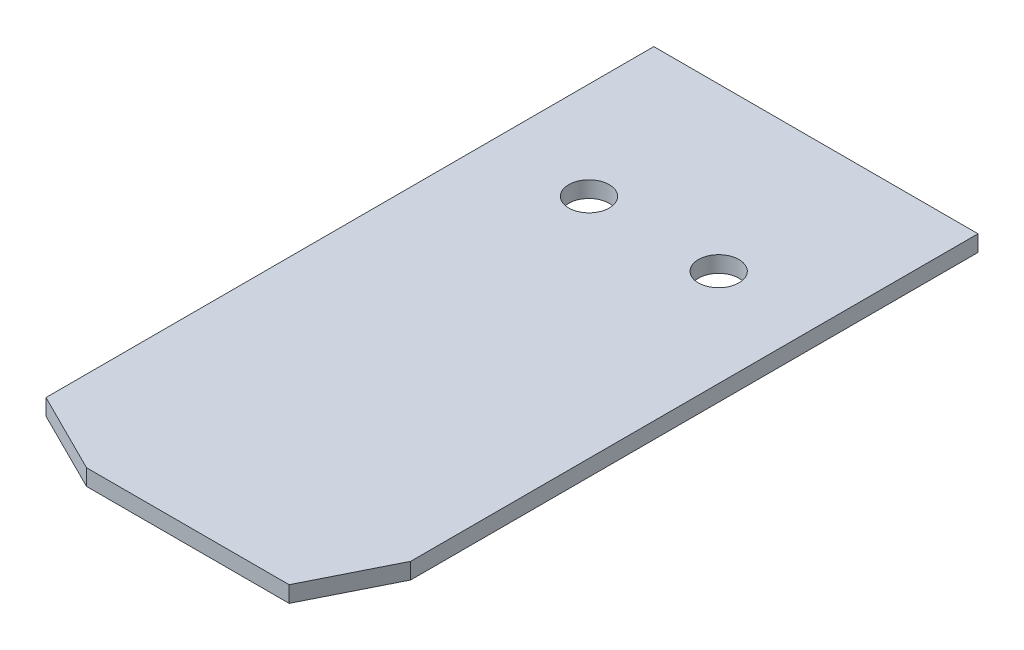
from build123d import *
from OCP.BRepFilletAPI import BRepFilletAPI_MakeChamfer

# Parameters (mm, degrees)
SKETCH1_W           = 40
SKETCH1_H           = 80
BOSS_EXTRUDE1_DEPTH = 2
SKETCH2_R           = 2.5
CUT_EXTRUDE1_DEPTH  = 10
CHAMFER1_SIZE       = 5
CHAMFER1_SIZE2      = 10


with BuildPart() as part:
    # Sketch1 → Boss-Extrude1 (new body)
    with BuildSketch(Plane(origin=(0, 0, 0), x_dir=(1, 0, 0), z_dir=(0, 1, 0))):
        Rectangle(SKETCH1_W, SKETCH1_H)
    extrude(amount=BOSS_EXTRUDE1_DEPTH)

    # Sketch2 → Cut-Extrude1 (cut)
    with BuildSketch(Plane.XZ):
        with Locations(Location((8, -20, 0), (0, 0, 270))):
            Circle(SKETCH2_R)
        with Locations(Location((-8, -20, 0), (0, 0, 270))):
            Circle(SKETCH2_R)
    extrude(amount=-CUT_EXTRUDE1_DEPTH, mode=Mode.SUBTRACT)

    # Chamfer1: one chamfer whose edges measure the first distance from different faces: ONE call of the kernel's chamfer builder (chamfer() names one face for all edges)
    chamfer1_edges_1 = [part.edges().sort_by_distance(p)[0] for p in [
        (20, 1, 40),
    ]]
    chamfer1_side_1 = [part.faces().sort_by_distance(p)[0] for p in [
        (0, 1, 40),
    ]]
    chamfer1_edges_2 = [part.edges().sort_by_distance(p)[0] for p in [
        (-20, 1, 40),
    ]]
    chamfer1_side_2 = [part.faces().sort_by_distance(p)[0] for p in [
        (-20, 1, 0),
    ]]
    chamfer1 = BRepFilletAPI_MakeChamfer(part.part.solid().wrapped)
    for e in chamfer1_edges_1:
        chamfer1.Add(CHAMFER1_SIZE, CHAMFER1_SIZE2, e.wrapped, chamfer1_side_1[0].wrapped)  # the first distance lies on this face
    for e in chamfer1_edges_2:
        chamfer1.Add(CHAMFER1_SIZE, CHAMFER1_SIZE2, e.wrapped, chamfer1_side_2[0].wrapped)  # the first distance lies on this face
    add(Compound.cast(chamfer1.Shape()), mode=Mode.REPLACE)


solid = part.part
